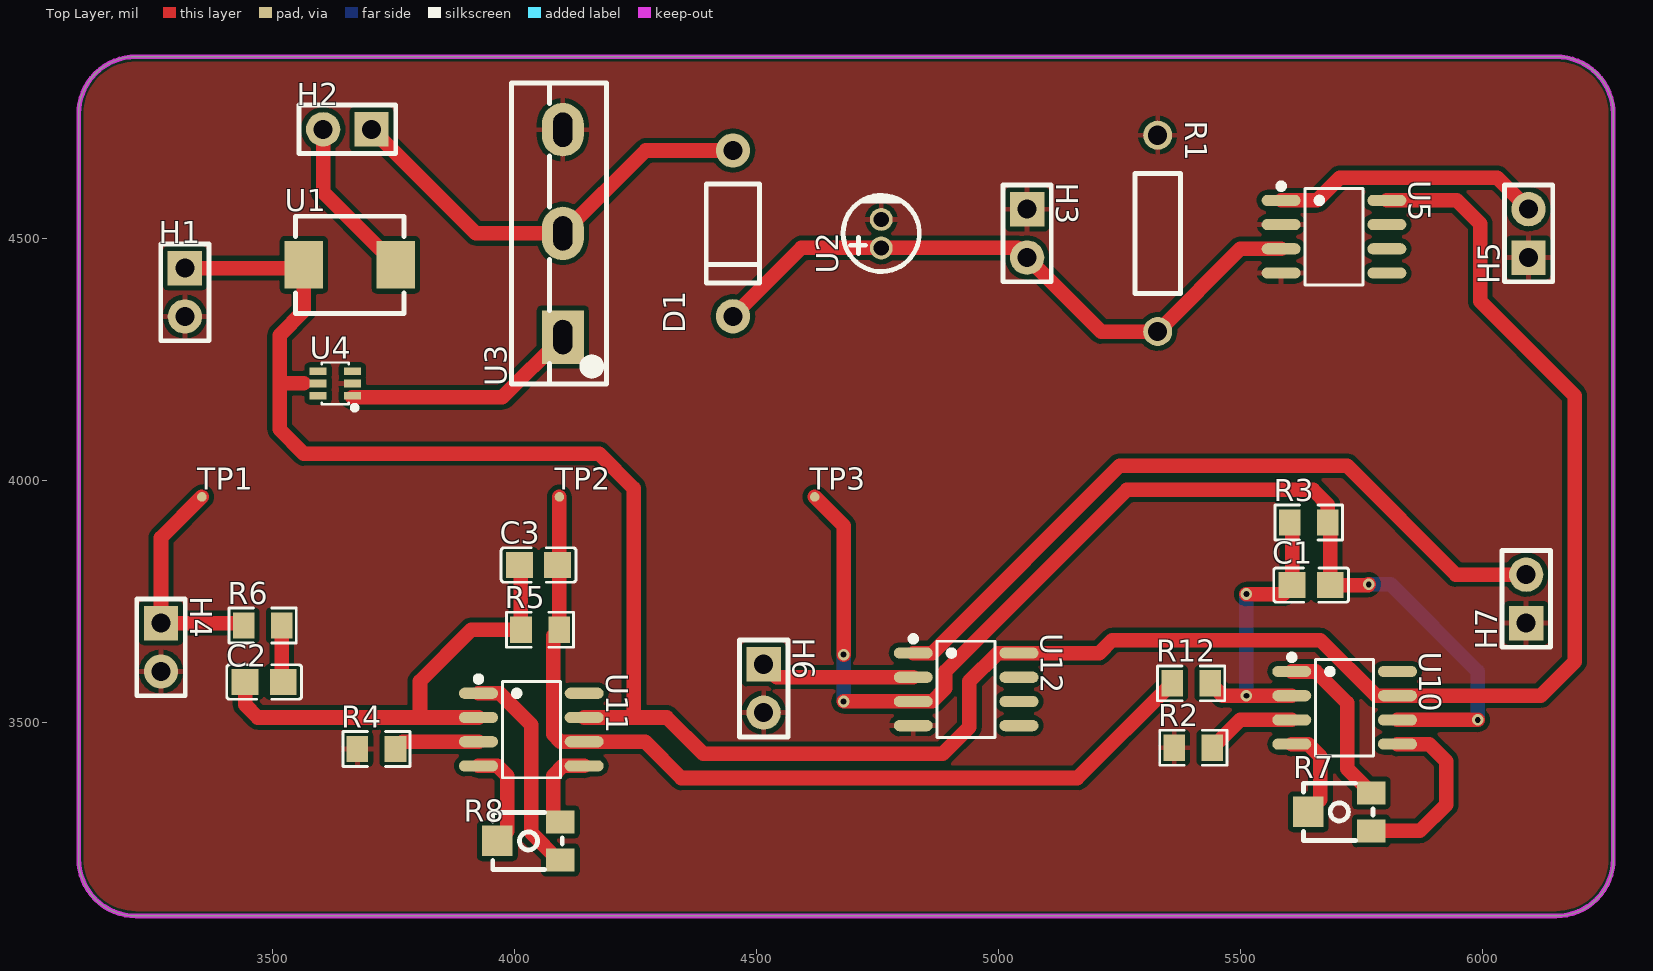
[diagram p0: Top Layer view]
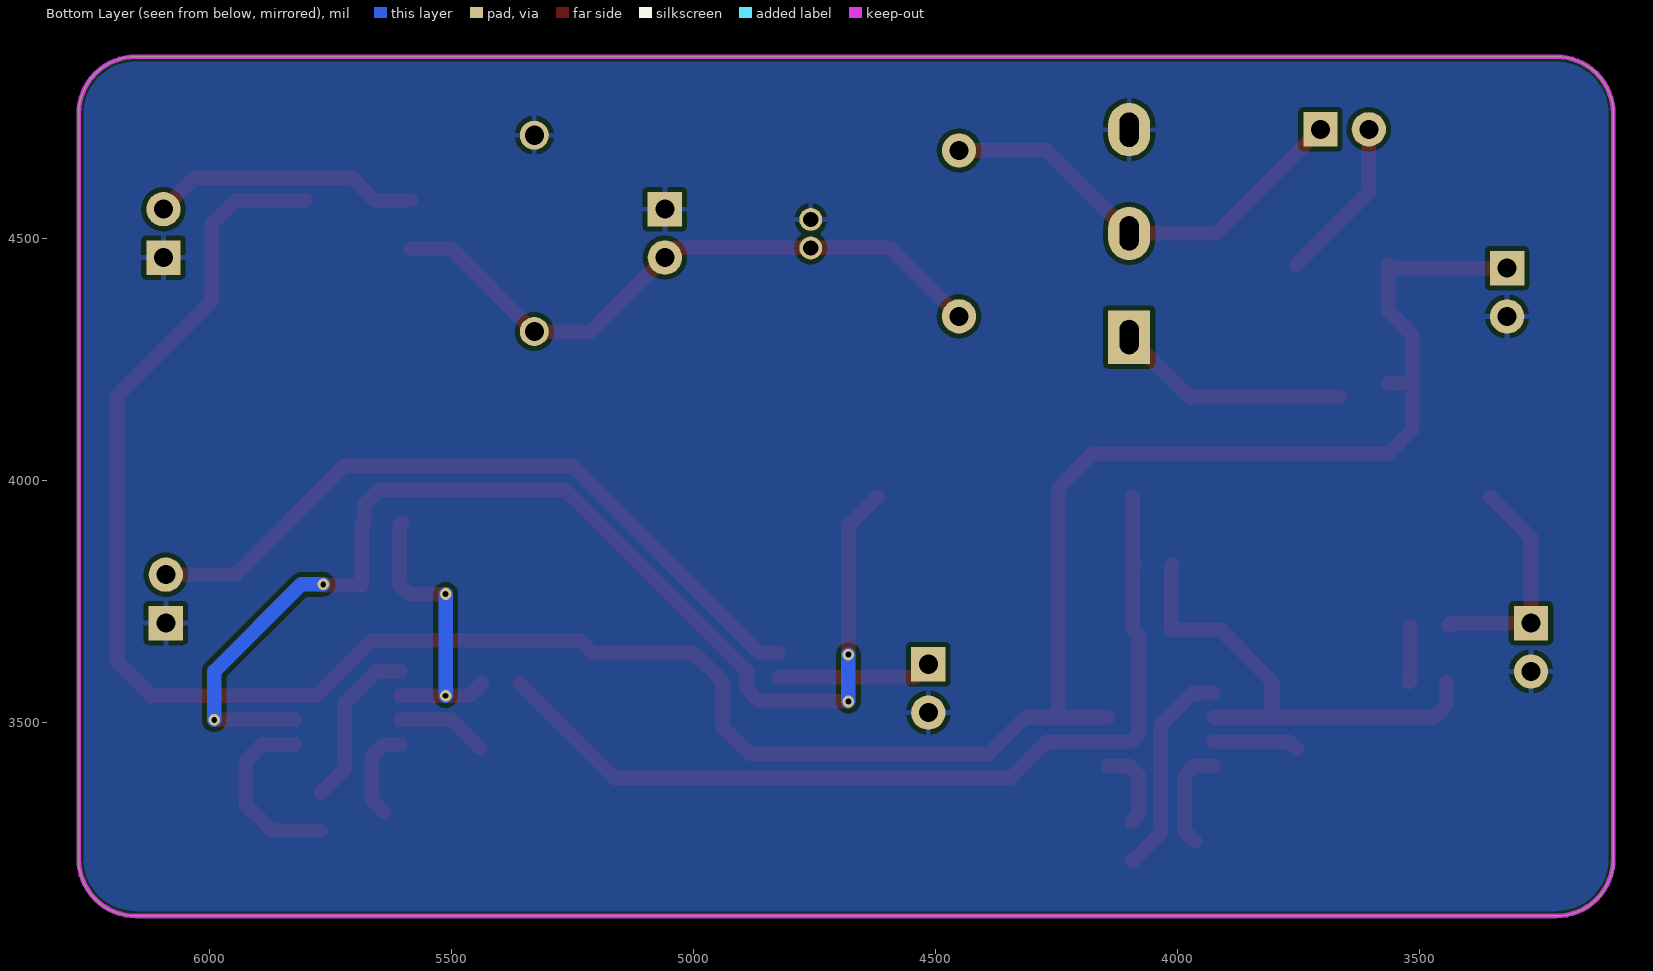
[diagram p1: Bottom Layer view, seen from below]
# Altium PCB MISC49892.pcbdoc
Units mil, origin at the board's own origin, x right, y up, seen from the top; angles counter-clockwise.
Board outline 3170 x 1775 mil, 2 copper layers (Top Layer, Bottom Layer), stack 62.206 mil thick; 31 components, 24 nets, 90 pads, 6 vias.

## Layer stack, top to bottom
Top Solder Mask Layer: solder mask 0.394, Dk 3.3
Top Layer: signal copper 1.379
Dielectric1: surface 59.449, FR4, Dk 4.5
Bottom Layer: signal copper 1.378
Bottom Solder Mask Layer: solder mask 0.394, Dk 3.3

## Board outline
3218.11,4875 ccw(c3218.11,4756.89) 3100,4756.89 3100,3218.11 ccw(c3218.11,3218.11) 3218.11,3100 6151.89,3100 ccw(c6151.89,3218.11) 6270,3218.11 6270,4756.89 ccw(c6151.89,4756.89) 6151.89,4875

## Design rules (kind name [scope] priority, off if disabled: settings)
BoardOutlineClearance copperThickness2oz_1 [All] p2 off: genericclearance=7.99 ignorepadtopadclearanceinfootprint=FALSE except(0: Arc-SplitContinuation Track-SplitContinuation SMDPad-SplitContinuation THPad-SplitContinuation Via-SplitContinuation Fill-SplitContinuation Region-SplitContinuation Poly-SplitContinuation Text-SplitContinuation Hole-SplitContinuation; 5.98: Arc-CutoutEdge Track-CutoutEdge SMDPad-CutoutEdge THPad-CutoutEdge Via-CutoutEdge Text-CutoutEdge; 6.9: Hole-OutlineEdge Hole-CutoutEdge; 10: Poly-OutlineEdge Poly-CutoutEdge; 11.81: Arc-OutlineEdge Track-OutlineEdge SMDPad-OutlineEdge THPad-OutlineEdge Via-OutlineEdge Fill-OutlineEdge Region-OutlineEdge Text-OutlineEdge Fill-CutoutEdge Region-CutoutEdge)
BoardOutlineClearance Plane_innerPlane_1 [All] p4 off: genericclearance=4.02 ignorepadtopadclearanceinfootprint=FALSE except(0: Arc-SplitContinuation Track-SplitContinuation SMDPad-SplitContinuation THPad-SplitContinuation Via-SplitContinuation Fill-SplitContinuation Region-SplitContinuation Poly-SplitContinuation Text-SplitContinuation Hole-SplitContinuation; 5.98: Arc-CutoutEdge Track-CutoutEdge SMDPad-CutoutEdge THPad-CutoutEdge Via-CutoutEdge Text-CutoutEdge; 6.9: Hole-OutlineEdge Hole-CutoutEdge; 10: Poly-OutlineEdge Poly-CutoutEdge; 11.81: Arc-OutlineEdge Track-OutlineEdge SMDPad-OutlineEdge THPad-OutlineEdge Via-OutlineEdge Fill-OutlineEdge Region-OutlineEdge Text-OutlineEdge Fill-CutoutEdge Region-CutoutEdge)
BoardOutlineClearance Copper_copperRegion_1 [All] p6 off: genericclearance=4.02 ignorepadtopadclearanceinfootprint=FALSE except(0: Arc-SplitContinuation Track-SplitContinuation SMDPad-SplitContinuation THPad-SplitContinuation Via-SplitContinuation Fill-SplitContinuation Region-SplitContinuation Poly-SplitContinuation Text-SplitContinuation Hole-SplitContinuation; 5.98: Arc-CutoutEdge Track-CutoutEdge SMDPad-CutoutEdge THPad-CutoutEdge Via-CutoutEdge Text-CutoutEdge; 6.9: Hole-OutlineEdge Hole-CutoutEdge; 10: Poly-OutlineEdge Poly-CutoutEdge; 11.81: Arc-OutlineEdge Track-OutlineEdge SMDPad-OutlineEdge THPad-OutlineEdge Via-OutlineEdge Fill-OutlineEdge Region-OutlineEdge Text-OutlineEdge Fill-CutoutEdge Region-CutoutEdge)
BoardOutlineClearance copperThickness1oz_1 [All] p8: genericclearance=4.02 ignorepadtopadclearanceinfootprint=FALSE except(0: Arc-SplitContinuation Track-SplitContinuation SMDPad-SplitContinuation THPad-SplitContinuation Via-SplitContinuation Fill-SplitContinuation Region-SplitContinuation Poly-SplitContinuation Text-SplitContinuation Hole-SplitContinuation; 5.98: Arc-CutoutEdge Track-CutoutEdge SMDPad-CutoutEdge THPad-CutoutEdge Via-CutoutEdge Text-CutoutEdge; 6.9: Hole-OutlineEdge Hole-CutoutEdge; 10: Poly-OutlineEdge Poly-CutoutEdge; 11.81: Arc-OutlineEdge Track-OutlineEdge SMDPad-OutlineEdge THPad-OutlineEdge Via-OutlineEdge Fill-OutlineEdge Region-OutlineEdge Text-OutlineEdge Fill-CutoutEdge Region-CutoutEdge)
Clearance copperThickness2oz [All] p1 off: gap=7.99 ignorepadtopadclearanceinfootprint=FALSE except(5.98: SMDPad-Track SMDPad-SMDPad THPad-Track SMDPad-THPad THPad-THPad Track-Via SMDPad-Via THPad-Via Via-Via Fill-SMDPad Region-SMDPad Fill-THPad Region-THPad Fill-Via Region-Via Fill-Fill Fill-Region Region-Region Arc-Track Arc-SMDPad Arc-THPad Arc-Via Fill-Arc Region-Arc Arc-Arc Text-Track SMDPad-Text Text-THPad Text-Via Fill-Text Region-Text Arc-Text Text-Text; 6.9: Hole-Track Hole-SMDPad Hole-THPad Hole-Via Fill-Hole Region-Hole Hole-Arc Hole-Text; 10: Poly-Track Poly-SMDPad Poly-THPad Poly-Via Poly-Fill Poly-Region Poly-Poly Poly-Arc Poly-Text Poly-Hole; 11.81: Fill-Track Region-Track)
Clearance Plane_innerPlane [All] p3 off: gap=4.02 ignorepadtopadclearanceinfootprint=FALSE except(5.98: SMDPad-Track SMDPad-SMDPad THPad-Track SMDPad-THPad THPad-THPad Track-Via SMDPad-Via THPad-Via Via-Via Fill-SMDPad Region-SMDPad Fill-THPad Region-THPad Fill-Via Region-Via Fill-Fill Fill-Region Region-Region Arc-Track Arc-SMDPad Arc-THPad Arc-Via Fill-Arc Region-Arc Arc-Arc Text-Track SMDPad-Text Text-THPad Text-Via Fill-Text Region-Text Arc-Text Text-Text; 6.9: Hole-Track Hole-SMDPad Hole-THPad Hole-Via Fill-Hole Region-Hole Hole-Arc Hole-Text; 10: Poly-Track Poly-SMDPad Poly-THPad Poly-Via Poly-Fill Poly-Region Poly-Poly Poly-Arc Poly-Text Poly-Hole; 11.81: Fill-Track Region-Track)
Clearance Copper_copperRegion [All] p5 off: gap=4.02 ignorepadtopadclearanceinfootprint=FALSE except(5.98: SMDPad-Track SMDPad-SMDPad THPad-Track SMDPad-THPad THPad-THPad Track-Via SMDPad-Via THPad-Via Via-Via Fill-SMDPad Region-SMDPad Fill-THPad Region-THPad Fill-Via Region-Via Fill-Fill Fill-Region Region-Region Arc-Track Arc-SMDPad Arc-THPad Arc-Via Fill-Arc Region-Arc Arc-Arc Text-Track SMDPad-Text Text-THPad Text-Via Fill-Text Region-Text Arc-Text Text-Text; 6.9: Hole-Track Hole-SMDPad Hole-THPad Hole-Via Fill-Hole Region-Hole Hole-Arc Hole-Text; 10: Poly-Track Poly-SMDPad Poly-THPad Poly-Via Poly-Fill Poly-Region Poly-Poly Poly-Arc Poly-Text Poly-Hole; 11.81: Fill-Track Region-Track)
Clearance copperThickness1oz [All] p7: gap=4.02 ignorepadtopadclearanceinfootprint=FALSE except(5.98: SMDPad-Track SMDPad-SMDPad THPad-Track SMDPad-THPad THPad-THPad Track-Via SMDPad-Via THPad-Via Via-Via Fill-SMDPad Region-SMDPad Fill-THPad Region-THPad Fill-Via Region-Via Fill-Fill Fill-Region Region-Region Arc-Track Arc-SMDPad Arc-THPad Arc-Via Fill-Arc Region-Arc Arc-Arc Text-Track SMDPad-Text Text-THPad Text-Via Fill-Text Region-Text Arc-Text Text-Text; 6.9: Hole-Track Hole-SMDPad Hole-THPad Hole-Via Fill-Hole Region-Hole Hole-Arc Hole-Text; 10: Poly-Track Poly-SMDPad Poly-THPad Poly-Via Poly-Fill Poly-Region Poly-Poly Poly-Arc Poly-Text Poly-Hole; 11.81: Fill-Track Region-Track)
DiffPairsRouting differentialPair [All] p1: maxlimit=6 minlimit=6 mostfreqgap=6 toplayer_minwidth=5 toplayer_prefwidth=10 toplayer_maxwidth=100 toplayer_mingap=6 toplayer_prefgap=6 toplayer_maxgap=6 bottomlayer_minwidth=5 bottomlayer_prefwidth=10 bottomlayer_maxwidth=100 bottomlayer_mingap=6 bottomlayer_prefgap=6 bottomlayer_maxgap=6 maxuncoupledlength=10
HoleToHoleClearance otherClearance [All] p1: gap=11.81 allowstackedmicrovias=TRUE
Length netLength [All] p1: minlimit=0 maxlimit=0
PasteMaskExpansion pasteMaskExpansion [All] p1: expansion=0
PlaneConnect innerPlane [All] p1: planeconnectstyle=Relief reliefexpansion=20 reliefentries=4 reliefconductorwidth=10 reliefairgap=10
PolygonConnect copperRegion [All] p1: connectstyle=Relief reliefconductorwidth=10 reliefentries=4 polygonreliefangle="90 Angle" airgapwidth=10 via.connectstyle=Relief via.reliefconductorwidth=10 via.reliefentries=4 via.polygonreliefangle="90 Angle" via.airgapwidth=10
RoutingVias viaSize [All] p1: holewidth=12.01 width=24.02 viastyle="Through Hole" minholewidth=11.81 minwidth=19.68 maxholewidth=248.03 maxwidth=393.7
SolderMaskExpansion solderMaskExpansion [IsVia] p1: expansion=-1000 istentingtop=TRUE
SolderMaskExpansion solderMaskExpansion [All] p2: expansion=2 istentingtop=FALSE
Width copperThickness2oz_2 [All] p1 off: maxlimit=100 minlimit=8 preferedwidth=10
Width copperThickness1oz_2 [All] p2: maxlimit=100 minlimit=5 preferedwidth=10

## Components (designator, comment, footprint, x,y, rotation, side; value= is the part's Value field where it differs from the comment)
C1 "100nF" C0805 5645.88,3783.59 r0 top
C2 "100nF" C0805 3483.1,3583.33 r180 top
C3 "1nF" C0805 4050,3825 r0 top
D1 "" DO_1N4007 4451.5,4510 r90 top
H1 "" HDR-TH_2P-P2.54-V-M-1 3319.36,4388.27 r270 top
H2 "" HDR-TH_2P-P2.54-V-M-1 3655,4725 r180 top
H3 "" HDR-TH_2P-P2.54-V-M-1 5059.14,4510 r270 top
H4 "" HDR-TH_2P-P2.54-V-M-1 3270,3655 r270 top
H5 "" HDR-TH_2P-P2.54-V-M-1 6095,4510 r90 top
H6 "" HDR-TH_2P-P2.54-V-M-1 4515,3570 r270 top
H7 "" HDR-TH_2P-P2.54-V-M-1 6090,3755 r90 top
R1 "10kΩ" Res_1/4W 5328.9,4510 r270 top
R2 "10kΩ" R0805 5402.41,3447.47 r0 top
R3 "1MΩ" R0805 5640.88,3912.79 r0 top
R4 "10kΩ" R0805 3715,3445 r0 top
R5 "10kΩ" R0805 4052.94,3691.23 r0 top
R6 "100Ω" R0805 3480,3700 r0 top
R7 "100kΩ" RES-ADJ-SMD_VG039NCH 5705,3315 r0 top
R8 "100kΩ" RES-ADJ-SMD_VG039NCH 4030,3255 r0 top
R12 "10kΩ" R0805 5398.06,3580.66 r0 top
TP1 "" Test-Point-0.5mm 3354.36,3965.8 r0 top
TP2 "" Test-Point-0.5mm 4092.94,3965.8 r0 top
TP3 "" Test-Point-0.5mm 4620.38,3965.8 r0 top
U1 "功率电感(贴片),CKST0502-10uH/M,10uH,±20%,3A,封装5.7mm*5.1mm*2.0mm,岑科,RoHS" IND-SMD_L5.7-W5.1 3660,4445 r0 top
U2 "10uF" CAP-TH_BD4.0-P1.50-D0.8-FD 4757.84,4509.4 r90 top
U3 "HY5204" TO-247-3_L15.8-W5.0-P5.44-L-1 4100,4510 r90 top
U4 "SN74LVC2G04DCKR" SOT-363_L2.0-W1.3-P0.65-LS2.1-BR 3630,4200 r0 top
U5 "NE5532DR" SOIC-8_L4.9-W3.9-P1.27-LS6.0-BL 5693.07,4503.13 r270 top
U10 "UA741CDT" SOIC-8_L4.9-W3.9-P1.27-LS6.0-BL 5715,3530 r270 top
U11 "UA741CDT" SOIC-8_L4.9-W3.9-P1.27-LS6.0-BL 4035,3485 r270 top
U12 "NE5532DR" SOIC-8_L4.9-W3.9-P1.27-LS6.0-BL 4933.13,3568.13 r270 top

## Footprints (in the part's own frame and the unit in brackets; to place one, negate y for a bottom-side part, rotate by r counter-clockwise, add the part's x,y. Pads: shape width x height; smd on the part's side, far side on the other; paste and mask are expansions set on the pad)
C0805 [mm]
  rect 1.41x1.35 smd paste-100 mask+0.051: 1(-1,0) 2(1,0)
  silkscreen extent -1.96,-0.9 1.96,0.9
CAP-TH_BD4.0-P1.50-D0.8-FD [mm]
  round 1.2 hole 0.8: 1(-0.75,0) 2(0.75,0)
  silkscreen extent -1.98,-2 2.06,2
DO_1N4007 [mm]
  round 1.8 hole 1 paste+0 mask+0.051: 1(-4.35,0) 2(4.35,0)
  silkscreen extent -2.6,-1.4 2.6,1.4
HDR-TH_2P-P2.54-V-M-1 [mm]
  rect 1.8x1.8 hole 1: 1(-1.27,0)
  round 1.8 hole 1: 2(1.27,0)
  silkscreen extent -2.54,-1.27 2.54,1.27
IND-SMD_L5.7-W5.1 [mm]
  rect 2x2.5 smd paste+0 mask+0.05: 1(-2.413,0) 2(2.413,0)
  silkscreen extent -2.85,-2.55 2.85,2.55
R0805 [mm]
  rect 1.133x1.377 smd paste-100 mask+0.051: 1(-1,0) 2(1,0)
  silkscreen extent -1.76,-0.92 1.76,0.92
RES-ADJ-SMD_VG039NCH [mm]
  rect 1.5x1.2 smd: 1(1.65,-1) 3(1.65,1)
  rect 1.6x1.6 smd: 2(-1.65,0)
  silkscreen extent -1.9,-1.5 1.75,1.5
Res_1/4W [mil]
  round 60 hole 39.37 paste+0 mask+2: 1(-202.76,0) 2(202.76,0)
  silkscreen extent -124,-47 124,47
SOIC-8_L4.9-W3.9-P1.27-LS6.0-BL [mm]
  oval 0.588x2.045 smd: 1(-1.905,-2.772) 2(-0.635,-2.772) 3(0.635,-2.772) 4(1.905,-2.772) 5(1.905,2.772) 6(0.635,2.772) 7(-0.635,2.772) 8(-1.905,2.772)
  silkscreen extent -2.8,-2.92 2.53,1.52
SOT-363_L2.0-W1.3-P0.65-LS2.1-BR [mm]
  rect 0.9x0.4 smd: 1(0.9,-0.65) 2(0.9,0) 3(0.9,0.65) 4(-0.9,0.65) 5(-0.9,0) 6(-0.9,-0.65)
  silkscreen extent -0.7,-1.4 1.14,1.1
Test-Point-0.5mm [mm]
  round 0.5 smd: 1(0,0)
TO-247-3_L15.8-W5.0-P5.44-L-1 [mm]
  rect 2.8x2.2 hole 1 slot 1.8 at 0 deg paste+0 mask+0.05: 1(-5.44,0)
  oval 2.8x2.2 hole 1 slot 1.8 at 0 deg paste+0 mask+0.05: 2(0,0) 3(5.44,0)
  silkscreen extent -7.9,-2.3 7.9,2.7

## Via types
v1: diameter 24, hole 12, Top Layer to Bottom Layer, 5 vias
v2: diameter 24.02, hole 12, Top Layer to Bottom Layer, 1 vias

## Nets (pads, with @x,y where several pads share a name; then routed paths per layer and width w, separated by ;. In a path a pad name is that pad's centre, name@x,y a point inside that pad or via, vN(x,y) a via of type N, cw(c..) or ccw(c..) an arc to the next point about the centre after c; other vN are vias at no path point)
$1N178: H2.2 U1.2 | length 342.1
  Top Layer w30: H2.2 3605,4595 U1.2
$1N206: D1.2 H2.1 U3.2 | length 906.5
  Top Layer w30: H2.1 3920,4510 U3.2 4271.26,4681.26 D1.2
$1N266: D1.1 H3.2 R1.2 U2.1 U5.3 | length 1333.2
  Top Layer w30: D1.1 4592.63,4479.87 U2.1 5039.27,4479.87 H3.2 5211.9,4307.24 R1.2 5499.79,4478.13 U5.3
$1N648: U3.1 U4.1 | length 486.2
  Top Layer w30: U4.1@3665.43,4171.15 3975.32,4171.15 U3.1
$1N1018: H4.1 R6.1 TP1.1 | length 468.4
  Top Layer w30: TP1.1 3270,3881.44 H4.1 3435.63,3705 R6.1
$1N3426: R7.3 U10.1 | length 347.4
  Top Layer w30: U10.1 5655,3605 5720,3540 5720,3404.33 R7.3
$1N3427: R7.1 U10.5 | length 382.9
  Top Layer w30: R7.1 5870.63,3275.63 5925,3330 5925,3420 5890,3455 U10.5
$1N3428: R2.2 U10.3 | length 187.9
  Top Layer w30: R2.2 5499.32,3505 U10.3
$1N3429: C1.1 R3.1 R12.2 U10.2 | length 622.5
  Top Layer w30: R12.2 5463.09,3555 v2(5512.02,3555) U10.2 ; v1(5512.02,3765) 5587.92,3765 C1.1 5606.51,3907.79 R3.1
  Bottom Layer w30: v2(5512.02,3555) v1(5512.02,3765)
$1N3432: C1.2 R3.2 TP3.1 U10.6 U12.3 | length 2475.6
  Top Layer w30: TP3.1 4680,3906.17 v1(4680,3640) ; v1(4680,3543.13) U12.3 4863.13,3543.13 4890,3570 4890,3605 5265,3980 5650,3980 5680.25,3949.75 R3.2 5685.25,3907.79 C1.2 5763.59,3783.59 v1(5765,3785) ; U10.6 v1(5990,3505)
  Bottom Layer w30: v1(4680,3543.13) v1(4680,3640) ; v1(5765,3785) 5810,3785 5990,3605 v1(5990,3505)
$1N3433: C3.2 R5.2 R12.1 TP2.1 U11.6 | length 1895.6
  Top Layer w30: TP2.1 4092.94,3828.57 C3.2 4092.31,3822.06 R5.2 4080,3678.92 4080,3475 4095,3460 U11.6 4270,3460 4345,3385 5163.02,3385 R12.1
$1N3435: C2.1 R6.2 | length 118
  Top Layer w30: R6.2 3519.37,3586.43 C2.1
$1N3436: R4.2 U11.3 | length 177.7
  Top Layer w30: R4.2 3769.37,3460 U11.3
$1N3437: R8.1 U11.1 | length 442.7
  Top Layer w30: U11.1 3970,3560 4035,3495 4035,3271.51 4090.88,3215.63 R8.1
$1N3439: R8.3 U11.5 | length 174.3
  Top Layer w30: R8.3 4080,3309.33 4080,3390 4100,3410 U11.5
$1N3440: C2.2 C3.1 R5.1 U11.2 | length 1006.1
  Top Layer w30: C2.2 3443.73,3536.27 3470,3510 3796.55,3510 ; U11.2 3796.55,3510 ; C3.1 4013.57,3822.06 R5.1 3911.23,3691.23 3805,3585 3805,3518.45 3796.55,3510
$1N3876: H6.1 U12.2 | length 320.1
  Top Layer w30: H6.1 4541.87,3593.13 U12.2
-9V: R8.2 U11.4 | length 210.7
  Top Layer w30: U11.4 3965,3410 3985,3390 3985,3274.96 R8.2
-VCC: R7.2 U10.4 | length 194.8
  Top Layer w30: U10.4 5640,3455 5665,3430 5665,3339.96 R7.2
GND: H1.2 H3.1 H4.2 H5.1 H6.2 H7.1 R1.1 R2.1 R4.1 U2.2 U3.3 U4.2 U5.2 U5.4 U12.4
V0: U4.6
VC: H7.2 U12.1 | length 1519.5
  Top Layer w30: U12.1 4863.13,3643.13 5250,4030 5720,4030 5945,3805 H7.2
VCC: H1.1 U1.1 U4.5 U5.8 U10.7 U11.7 U12.8 | length 5419.7
  Top Layer w30: H1.1 3558.27,4438.27 U1.1 3565,4350 3515,4300 3515,4200.49 ; 3564.89,4200 3564.4,4200.49 3515,4200.49 ; U11.7 4246.89,3510 ; U5.8 5946.87,4578.13 5995,4530 5995,4370 6190,4175 6190,3625 6120,3555 U10.7 5780,3555 5665,3670 5235,3670 5208.13,3643.13 U12.8 4998.13,3643.13 4940,3585 4940,3490 4885,3435 4390,3435 4315,3510 4246.89,3510 ; 3515,4200.49 3515,4105 3565,4055 4175,4055 4246.89,3983.11 4246.89,3510
VOUT: H5.2 U5.1 | length 557.4
  Top Layer w30: U5.1 5658.13,4578.13 5705,4625 6030,4625 H5.2
pads on no net: U4.3 U4.4 U5.5 U5.6 U5.7 U10.8 U11.8 U12.5 U12.6 U12.7

## Polygon pours and split planes (outlines as drawn)
GND on Top Layer (solid, remove dead copper, pour order 0): 3000,5015 3000,3000 6400,3000 6400,5015
GND on Bottom Layer (solid, remove dead copper, pour order 2): 3055,4995 3055,3025 6390,3025 6390,4995

## Keep-outs
Board Outline Layer:
  the board outline again, w10